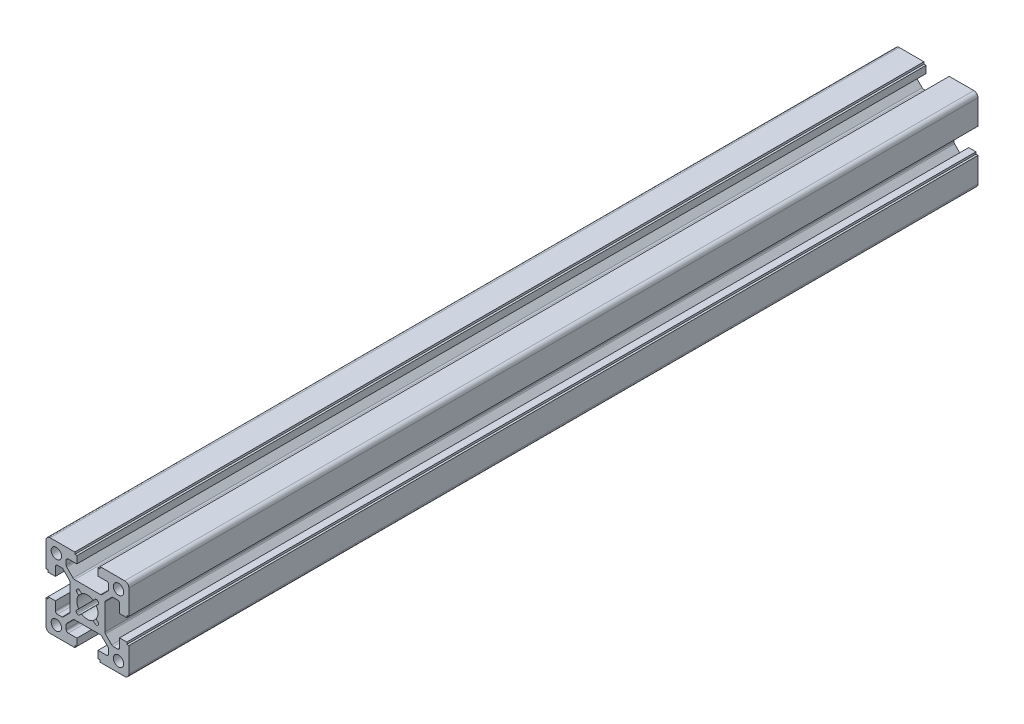
from build123d import *

# Parameters (mm, degrees)
SKETCH1_R           = 2.5
BOSS_EXTRUDE1_DEPTH = 205


with BuildPart() as part:
    # Sketch1 → Boss-Extrude1 (new, symmetric)
    with BuildSketch(Plane.XY):
        with BuildLine():
            Line((-5.1005, 15.500896213), (-5.1005, 19.000896213))
            Line((-5.1005, 19.000896213), (-6.1005, 19.000896213))
            Line((-6.1005, 19.000896213), (-6.1005, 20.000896213))
            Line((-6.1005, 20.000896213), (-18.0005, 20.000896213))
            ThreePointArc((-18.0005, 20.000896213), (-19.414713562, 19.415109775), (-20.0005, 18.000896213))
            Line((-20.0005, 18.000896213), (-20.0005, 6.100896213))
            Line((-20.0005, 6.100896213), (-19.0005, 6.100896213))
            Line((-19.0005, 6.100896213), (-19.0005, 5.100896213))
            Line((-19.0005, 5.100896213), (-15.5005, 5.100896213))
            Line((-15.5005, 5.100896213), (-15.5005, 9.250896213))
            ThreePointArc((-15.5005, 9.250896213), (-15.207606781, 9.958002994), (-14.5005, 10.250896213))
            Line((-14.5005, 10.250896213), (-12.431713562, 10.250896213))
            ThreePointArc((-12.431713562, 10.250896213), (-12.049030228, 10.174775786), (-11.724606932, 9.958003144))
            Line((-11.724606932, 9.958003144), (-8.693393219, 6.926789431))
            ThreePointArc((-8.693393219, 6.926789431), (-8.476620546, 6.602366272), (-8.4005, 6.21968306))
            Line((-8.4005, 6.21968306), (-8.4005, -6.217890225))
            ThreePointArc((-8.4005, -6.217890225), (-8.476620502, -6.60057374), (-8.693393346, -6.924997133))
            Line((-8.693393346, -6.924997133), (-11.724606781, -9.956210569))
            ThreePointArc((-11.724606781, -9.956210569), (-12.049030198, -10.172983348), (-12.431713709, -10.249103787))
            Line((-12.431713709, -10.249103787), (-14.5005, -10.249103787))
            ThreePointArc((-14.5005, -10.249103787), (-15.207606781, -9.956210569), (-15.5005, -9.249103787))
            Line((-15.5005, -9.249103787), (-15.5005, -5.099103787))
            Line((-15.5005, -5.099103787), (-19.0005, -5.099103787))
            Line((-19.0005, -5.099103787), (-19.0005, -6.099103787))
            Line((-19.0005, -6.099103787), (-20.0005, -6.099103787))
            Line((-20.0005, -6.099103787), (-20.0005, -17.999103787))
            ThreePointArc((-20.0005, -17.999103787), (-19.414713562, -19.41331735), (-18.0005, -19.999103787))
            Line((-18.0005, -19.999103787), (-6.1005, -19.999103787))
            Line((-6.1005, -19.999103787), (-6.1005, -18.999103787))
            Line((-6.1005, -18.999103787), (-5.1005, -18.999103787))
            Line((-5.1005, -18.999103787), (-5.1005, -15.499103787))
            Line((-5.1005, -15.499103787), (-9.2505, -15.499103787))
            ThreePointArc((-9.2505, -15.499103787), (-9.957606781, -15.206210569), (-10.2505, -14.499103787))
            Line((-10.2505, -14.499103787), (-10.2505, -12.43131735))
            ThreePointArc((-10.2505, -12.43131735), (-10.174379535, -12.048633922), (-9.957606789, -11.724210576))
            Line((-9.957606789, -11.724210576), (-6.925393219, -8.691997006))
            ThreePointArc((-6.925393219, -8.691997006), (-6.60096987, -8.475224255), (-6.218286438, -8.399103787))
            Line((-6.218286438, -8.399103787), (6.218286438, -8.399103787))
            ThreePointArc((6.218286438, -8.399103787), (6.600969772, -8.475224214), (6.925393068, -8.691996856))
            Line((6.925393068, -8.691996856), (9.956606781, -11.723210569))
            ThreePointArc((9.956606781, -11.723210569), (10.173379454, -12.047633728), (10.2495, -12.43031694))
            Line((10.2495, -12.43031694), (10.2495, -14.499103787))
            ThreePointArc((10.2495, -14.499103787), (9.956606781, -15.206210569), (9.2495, -15.499103787))
            Line((9.2495, -15.499103787), (5.0995, -15.499103787))
            Line((5.0995, -15.499103787), (5.0995, -18.999103787))
            Line((5.0995, -18.999103787), (6.0995, -18.999103787))
            Line((6.0995, -18.999103787), (6.0995, -19.999103787))
            Line((6.0995, -19.999103787), (17.9995, -19.999103787))
            ThreePointArc((17.9995, -19.999103787), (19.413713562, -19.41331735), (19.9995, -17.999103787))
            Line((19.9995, -17.999103787), (19.9995, -6.099103787))
            Line((19.9995, -6.099103787), (18.9995, -6.099103787))
            Line((18.9995, -6.099103787), (18.9995, -5.099103787))
            Line((18.9995, -5.099103787), (15.4995, -5.099103787))
            Line((15.4995, -5.099103787), (15.4995, -9.249103787))
            ThreePointArc((15.4995, -9.249103787), (15.206606781, -9.956210569), (14.4995, -10.249103787))
            Line((14.4995, -10.249103787), (12.431713562, -10.249103787))
            ThreePointArc((12.431713562, -10.249103787), (12.049030135, -10.172983322), (11.724606789, -9.956210576))
            Line((11.724606789, -9.956210576), (8.692393219, -6.923997006))
            ThreePointArc((8.692393219, -6.923997006), (8.475620467, -6.599573657), (8.3995, -6.216890225))
            Line((8.3995, -6.216890225), (8.3995, 6.21868265))
            ThreePointArc((8.3995, 6.21868265), (8.475620465, 6.601366078), (8.692393211, 6.925789424))
            Line((8.692393211, 6.925789424), (11.724606781, 9.958002994))
            ThreePointArc((11.724606781, 9.958002994), (12.04903013, 10.174775745), (12.431713562, 10.250896213))
            Line((12.431713562, 10.250896213), (14.4995, 10.250896213))
            ThreePointArc((14.4995, 10.250896213), (15.206606781, 9.958002994), (15.4995, 9.250896213))
            Line((15.4995, 9.250896213), (15.4995, 5.100896213))
            Line((15.4995, 5.100896213), (18.9995, 5.100896213))
            Line((18.9995, 5.100896213), (18.9995, 6.100896213))
            Line((18.9995, 6.100896213), (19.9995, 6.100896213))
            Line((19.9995, 6.100896213), (19.9995, 18.000896213))
            ThreePointArc((19.9995, 18.000896213), (19.413713562, 19.415109775), (17.9995, 20.000896213))
            Line((17.9995, 20.000896213), (6.0995, 20.000896213))
            Line((6.0995, 20.000896213), (6.0995, 19.000896213))
            Line((6.0995, 19.000896213), (5.0995, 19.000896213))
            Line((5.0995, 19.000896213), (5.0995, 15.500896213))
            Line((5.0995, 15.500896213), (9.2495, 15.500896213))
            ThreePointArc((9.2495, 15.500896213), (9.956606781, 15.208002994), (10.2495, 14.500896213))
            Line((10.2495, 14.500896213), (10.2495, 12.432109775))
            ThreePointArc((10.2495, 12.432109775), (10.173379498, 12.04942626), (9.956606654, 11.725002867))
            Line((9.956606654, 11.725002867), (6.925393219, 8.693789431))
            ThreePointArc((6.925393219, 8.693789431), (6.600969802, 8.477016652), (6.218286291, 8.400896213))
            Line((6.218286291, 8.400896213), (-6.218286438, 8.400896213))
            ThreePointArc((-6.218286438, 8.400896213), (-6.600969865, 8.477016678), (-6.925393211, 8.693789424))
            Line((-6.925393211, 8.693789424), (-9.957606781, 11.726002994))
            ThreePointArc((-9.957606781, 11.726002994), (-10.174379533, 12.050426343), (-10.2505, 12.433109775))
            Line((-10.2505, 12.433109775), (-10.2505, 14.500896213))
            ThreePointArc((-10.2505, 14.500896213), (-9.957606781, 15.208002994), (-9.2505, 15.500896213))
            Line((-9.2505, 15.500896213), (-5.1005, 15.500896213))
        make_face()
        with Locations((-15.0005, 15.000896213)):
            Circle(SKETCH1_R, mode=Mode.SUBTRACT)
        with Locations((14.9995, -14.999103787)):
            Circle(SKETCH1_R, mode=Mode.SUBTRACT)
        with Locations((-15.0005, -14.999103787)):
            Circle(SKETCH1_R, mode=Mode.SUBTRACT)
        with Locations((14.9995, 15.000896213)):
            Circle(SKETCH1_R, mode=Mode.SUBTRACT)
        with BuildLine():
            Line((-5.179163629, 3.765559841), (-4.2435, 2.829896213))
            ThreePointArc((-4.2435, 2.829896213), (-5.100062832, 0.000896213), (-4.2435, -2.828103787))
            Line((-4.2435, -2.828103787), (-5.277169914, -3.861773701))
            ThreePointArc((-5.277169914, -3.861773701), (-5.496839828, -4.392103787), (-5.277169914, -4.922433873))
            Line((-5.277169914, -4.922433873), (-4.923994614, -5.275609174))
            ThreePointArc((-4.923994614, -5.275609174), (-4.393905685, -5.495279049), (-3.8636756, -5.275950112))
            Line((-3.8636756, -5.275950112), (-2.8295, -4.243103787))
            ThreePointArc((-2.8295, -4.243103787), (0, -5.1), (2.8295, -4.243103787))
            Line((2.8295, -4.243103787), (3.778597046, -5.192200834))
            ThreePointArc((3.778597046, -5.192200834), (4.308685975, -5.411870709), (4.83891606, -5.192541772))
            Line((4.83891606, -5.192541772), (5.192983438, -4.838929494))
            ThreePointArc((5.192983438, -4.838929494), (5.412994471, -4.308499627), (5.193324596, -3.777928383))
            Line((5.193324596, -3.777928383), (4.2435, -2.828103787))
            ThreePointArc((4.2435, -2.828103787), (5.100062832, 0.000896213), (4.2435, 2.829896213))
            Line((4.2435, 2.829896213), (5.193264407, 3.77966062))
            ThreePointArc((5.193264407, 3.77966062), (5.412934321, 4.309990706), (5.193264407, 4.840320791))
            Line((5.193264407, 4.840320791), (4.839313907, 5.194271291))
            ThreePointArc((4.839313907, 5.194271291), (4.308742664, 5.413941166), (3.778312797, 5.193930133))
            Line((3.778312797, 5.193930133), (2.8295, 4.243896213))
            ThreePointArc((2.8295, 4.243896213), (0, 5.100792425), (-2.8295, 4.243896213))
            Line((-2.8295, 4.243896213), (-3.765163629, 5.179559841))
            ThreePointArc((-3.765163629, 5.179559841), (-4.295493715, 5.399229756), (-4.825823801, 5.179559841))
            Line((-4.825823801, 5.179559841), (-5.179163629, 4.826220013))
            ThreePointArc((-5.179163629, 4.826220013), (-5.398833543, 4.295889927), (-5.179163629, 3.765559841))
        make_face(mode=Mode.SUBTRACT)
    extrude(amount=BOSS_EXTRUDE1_DEPTH, both=True)


solid = part.part
